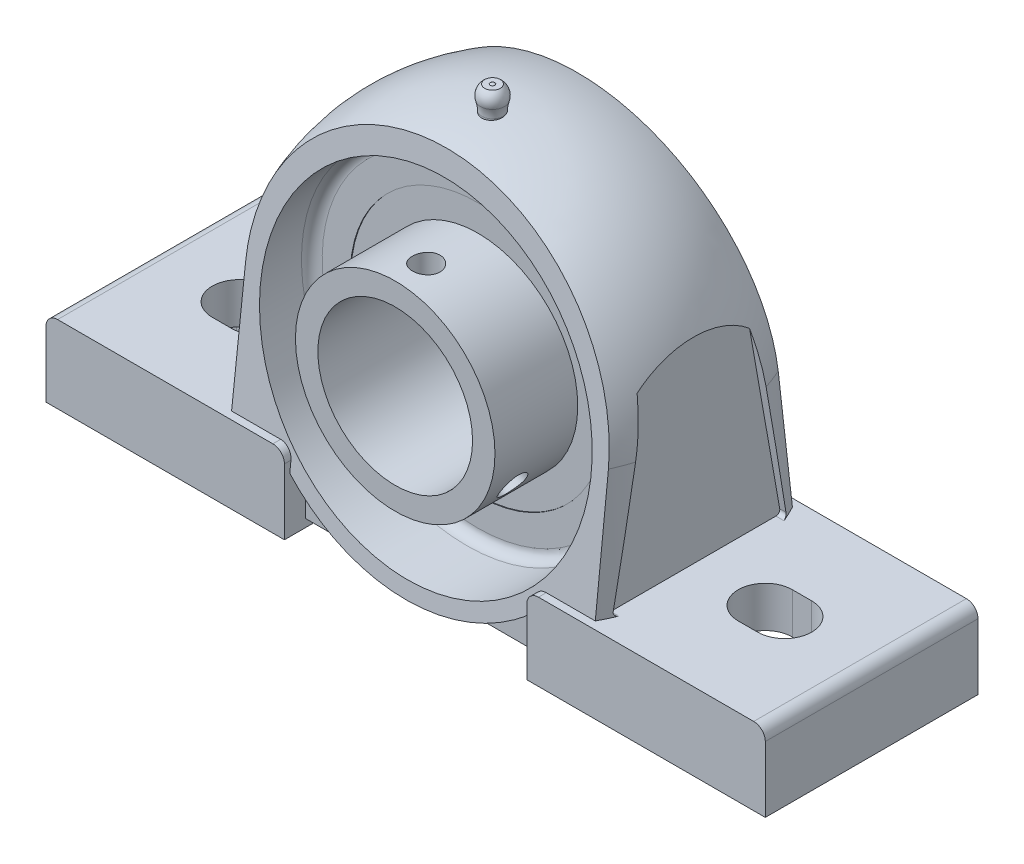
from build123d import *

# Parameters (mm, degrees)
BOSS_EXTRUDE_DEPTH              = 122.2
CUT_EXTRUDE1_DEPTH              = 80.400476324
CUT_EXTRUDE1_DEPTH_BACK         = 80.400476324
SKETCH5_OUTSIDE_W               = 85.446
SKETCH5_OUTSIDE_H               = 131.996
BOSS_EXTRUDE4_REACH             = 85.424
BOSS_EXTRUDE4_DIRECTION_2_REACH = 85.424
BOSS_EXTRUDE1_DEPTH             = 27.5
BOSS_EXTRUDE1_DEPTH_BACK        = 27.5
CUT_EXTRUDE3_DEPTH              = 145.261879946
CUT_EXTRUDE4_DEPTH              = 9.4
CUT_EXTRUDE4_DRAFT              = -1
CUT_EXTRUDE4_PROFILE_2_DEPTH    = 9.4
CUT_EXTRUDE4_PROFILE_2_DRAFT    = -1
CIRPATTERN1_COUNT               = 15
SKETCH14_W                      = 49.2
SKETCH14_H                      = 5.8
SKETCH16_W                      = 3.567
SKETCH16_H                      = 8
SKETCH15_W                      = 0.1
SKETCH15_H                      = 7.42
CIRPATTERN2_COUNT               = 2
CIRPATTERN2_ANGLE               = 120
CUT_EXTRUDE5_START              = 46.88824
CUT_EXTRUDE5_DEPTH              = 7.51176
CUT_EXTRUDE6_START              = -54.4
CUT_EXTRUDE6_DEPTH              = 7.50698


with BuildPart() as part:
    # Sketch1 → Boss-Extrude (new body)
    with BuildSketch(Plane(origin=(0, -47.2, 0), x_dir=(-1, 0, 0), z_dir=(0, 1, 0))):
        with BuildLine():
            Line((-47.716290457, 26.125), (47.716290457, 26.125))
            ThreePointArc((47.716290457, 26.125), (54.4, 0), (47.716290457, -26.125))
            Line((47.716290457, -26.125), (-47.716290457, -26.125))
            ThreePointArc((-47.716290457, -26.125), (-54.4, 0), (-47.716290457, 26.125))
        make_face()
    extrude(amount=BOSS_EXTRUDE_DEPTH)

    # Cut-Sweep1: sweep along a path in Sketch3
    with BuildLine(Plane.XY) as cut_sweep1_path:
        Line((-54.4, -47.2), (-51.514864415, 2.96289458))
        ThreePointArc((-51.514864415, 2.96289458), (0, 51.6), (51.514864415, 2.96289458))
        Line((51.514864415, 2.96289458), (54.4, -47.2))
    # Sketch2 → Cut-Sweep1 (sweep, cut)
    with BuildSketch(Plane(origin=(0, -47.2, 0), x_dir=(-1, 0, 0), z_dir=(0, 1, 0))):
        with BuildLine():
            Line((-47.716290457, 26.125), (-176.6, 26.125))
            Line((-176.6, 26.125), (-176.6, -26.125))
            Line((-176.6, -26.125), (-47.716290457, -26.125))
            ThreePointArc((-47.716290457, -26.125), (-54.4, 0), (-47.716290457, 26.125))
        make_face()
    sweep(path=cut_sweep1_path.line, mode=Mode.SUBTRACT)

    # Sketch5 outside → Cut-Extrude1 (cut, two sides: drawn at the far end of the back side and taken through both)
    with BuildSketch(Plane(origin=(0, 0, 0), x_dir=(0, 0, -1), z_dir=(1, 0, 0)).offset(-CUT_EXTRUDE1_DEPTH_BACK)):
        with Locations((0, 2.2)):
            Rectangle(SKETCH5_OUTSIDE_W, SKETCH5_OUTSIDE_H)
        Polygon((16.5, 52.6), (26.125, -35), (22, -35), (22, -50.2), (-22, -50.2), (-22, -35), (-26.125, -35), (-16.5, 52.6), align=None, mode=Mode.SUBTRACT)
    extrude(amount=CUT_EXTRUDE1_DEPTH + CUT_EXTRUDE1_DEPTH_BACK, mode=Mode.SUBTRACT)

    # Sketch6 → Cut-Revolve2 (revolve, cut)
    with BuildSketch(Plane(origin=(0, 0, 0), x_dir=(0, 0, -1), z_dir=(1, 0, 0)), mode=Mode.PRIVATE) as cut_revolve2_sk:
        with BuildLine():
            Line((-31.413703787, 42.761904762), (-11.679047619, 42.761904762))
            ThreePointArc((-11.679047619, 42.761904762), (-9.78467488, 41.977229881), (-9, 40.082857143))
            Line((-9, 40.082857143), (-9, 38.97435054))
            ThreePointArc((-9, 38.97435054), (-7.684345691, 39.254946584), (-6.36, 39.491143311))
            Line((-6.36, 39.491143311), (-6.36, 42.761904762))
            Line((-6.36, 42.761904762), (-3.72, 42.761904762))
            Line((-3.72, 42.761904762), (-3.72, 39.826644348))
            ThreePointArc((-3.72, 39.826644348), (2.674172991, 39.910509879), (9, 38.97435054))
            Line((9, 38.97435054), (9, 40.082857143))
            ThreePointArc((9, 40.082857143), (9.78467488, 41.977229881), (11.679047619, 42.761904762))
            Line((11.679047619, 42.761904762), (31.413703787, 42.761904762))
            Line((31.413703787, 42.761904762), (36.112143665, 0))
            Line((36.112143665, 0), (-36.112143665, 0))
            Line((-36.112143665, 0), (-31.413703787, 42.761904762))
        make_face()
    revolve(cut_revolve2_sk.sketch.rotate(Axis((0, 0, 0), (0, 0, -1)), 180), axis=Axis((0, 0, 0), (0, 0, -1)), mode=Mode.SUBTRACT)

    # Sketch11 → Boss-Revolve1 (revolve)
    with BuildSketch(Plane.XY.offset(5.04)):
        with BuildLine():
            Line((0, 48.911279127), (0, 57.6))
            ThreePointArc((0, 57.6), (-0.328456711, 57.530107141), (-0.6, 57.332539267))
            Line((-0.6, 57.332539267), (-2, 57.332539267))
            ThreePointArc((-2, 57.332539267), (-3.100653507, 55.744684437), (-3.105555556, 53.812665525))
            ThreePointArc((-3.105555556, 53.812665525), (-2.83938828, 52.646746373), (-2.75, 51.454176785))
            Line((-2.75, 51.454176785), (-2.75, 48.911279127))
            Line((-2.75, 48.911279127), (0, 48.911279127))
        make_face()
    revolve(axis=Axis((0, 0, 5.04), (0, 1, 0)))

    # Boss-Extrude4: up to this plane
    boss_extrude4_end = Plane(origin=(-54.4, 52.6, -16.5), z_dir=(0, 0.10921715097101498, -0.9940179142921794))
    # Sketch9 → Boss-Extrude4 (add, up to the surface)
    with BuildSketch(Plane.XY, mode=Mode.PRIVATE) as boss_extrude4_sk1:
        with BuildLine():
            Line((24.567875343, -35), (31.341433126, -35))
            ThreePointArc((31.341433126, -35), (0, -46.981756357), (-31.341433126, -35))
            Line((-31.341433126, -35), (-24.567875343, -35))
            ThreePointArc((-24.567875343, -35), (0, -42.761904762), (24.567875343, -35))
        make_face()
    boss_extrude4_tool1 = split(extrude(boss_extrude4_sk1.sketch, amount=-BOSS_EXTRUDE4_REACH, mode=Mode.PRIVATE), bisect_by=boss_extrude4_end, keep=Keep.BOTH, mode=Mode.PRIVATE)
    add(boss_extrude4_tool1.solids().sort_by_distance((27.954654, -35.638177, 0))[0])

    # Boss-Extrude4 direction 2: up to this plane
    boss_extrude4_direction_2_end = Plane(origin=(-54.4, 52.6, 16.5), z_dir=(0, 0.10921715097101498, 0.9940179142921794))
    # Sketch9 → Boss-Extrude4 direction 2 (add, up to the surface)
    with BuildSketch(Plane.XY, mode=Mode.PRIVATE) as boss_extrude4_direction_2_sk1:
        with BuildLine():
            Line((24.567875343, -35), (31.341433126, -35))
            ThreePointArc((31.341433126, -35), (0, -46.981756357), (-31.341433126, -35))
            Line((-31.341433126, -35), (-24.567875343, -35))
            ThreePointArc((-24.567875343, -35), (0, -42.761904762), (24.567875343, -35))
        make_face()
    boss_extrude4_direction_2_tool1 = split(extrude(boss_extrude4_direction_2_sk1.sketch, amount=BOSS_EXTRUDE4_DIRECTION_2_REACH, mode=Mode.PRIVATE), bisect_by=boss_extrude4_direction_2_end, keep=Keep.BOTH, mode=Mode.PRIVATE)
    add(boss_extrude4_direction_2_tool1.solids().sort_by_distance((27.954654, -35.638177, 0))[0])

    # Sketch4 → Boss-Extrude1 (add, two sides: drawn at the far end of the back side and taken through both)
    with BuildSketch(Plane.XY.offset(-BOSS_EXTRUDE1_DEPTH_BACK)):
        with BuildLine():
            Line((34.341433126, -29.2), (90, -29.2))
            ThreePointArc((90, -29.2), (92.121320344, -30.078679656), (93, -32.2))
            Line((93, -32.2), (93, -49.2))
            Line((93, -49.2), (31.341433126, -49.2))
            Line((31.341433126, -49.2), (31.341433126, -32.2))
            ThreePointArc((31.341433126, -32.2), (32.220112782, -30.078679656), (34.341433126, -29.2))
        make_face()
        with BuildLine():
            Line((-90, -29.2), (-34.341433126, -29.2))
            ThreePointArc((-34.341433126, -29.2), (-32.220112782, -30.078679656), (-31.341433126, -32.2))
            Line((-31.341433126, -32.2), (-31.341433126, -49.2))
            Line((-31.341433126, -49.2), (-93, -49.2))
            Line((-93, -49.2), (-93, -32.2))
            ThreePointArc((-93, -32.2), (-92.121320344, -30.078679656), (-90, -29.2))
        make_face()
    extrude(amount=BOSS_EXTRUDE1_DEPTH + BOSS_EXTRUDE1_DEPTH_BACK)

    # Sketch7 → Cut-Extrude3 (cut, through all)
    with BuildSketch(Plane.XZ.offset(49.2)):
        with BuildLine():
            Line((-65.5, 7), (-70.5, 7))
            ThreePointArc((-70.5, 7), (-77.5, 0), (-70.5, -7))
            Line((-70.5, -7), (-65.5, -7))
            ThreePointArc((-65.5, -7), (-58.5, 0), (-65.5, 7))
        make_face()
        with BuildLine():
            Line((65.5, -7), (70.5, -7))
            ThreePointArc((70.5, -7), (77.5, 0), (70.5, 7))
            Line((70.5, 7), (65.5, 7))
            ThreePointArc((65.5, 7), (58.5, 0), (65.5, -7))
        make_face()
    extrude(amount=-CUT_EXTRUDE3_DEPTH, mode=Mode.SUBTRACT)


with BuildPart() as cut_extrude4_tool:
    # Sketch10 → Cut-Extrude4 (with draft: the straight prism first)
    with BuildSketch(Plane.XZ.offset(49.2)):
        with BuildLine():
            ThreePointArc((70.5, -14.41), (71.015492065, -13.165492065), (72.26, -12.65))
            Line((72.26, -12.65), (83.815, -12.65))
            ThreePointArc((83.815, -12.65), (85.059507935, -12.134507935), (85.575, -10.89))
            Line((85.575, -10.89), (85.575, 10.89))
            ThreePointArc((85.575, 10.89), (85.059507935, 12.134507935), (83.815, 12.65))
            Line((83.815, 12.65), (72.26, 12.65))
            ThreePointArc((72.26, 12.65), (71.015492065, 13.165492065), (70.5, 14.41))
            Line((70.5, 14.41), (70.5, 18.315))
            ThreePointArc((70.5, 18.315), (69.984507935, 19.559507935), (68.74, 20.075))
            Line((68.74, 20.075), (40.526433126, 20.075))
            ThreePointArc((40.526433126, 20.075), (39.281925191, 19.559507935), (38.766433126, 18.315))
            Line((38.766433126, 18.315), (38.766433126, -18.315))
            ThreePointArc((38.766433126, -18.315), (39.281925191, -19.559507935), (40.526433126, -20.075))
            Line((40.526433126, -20.075), (68.74, -20.075))
            ThreePointArc((68.74, -20.075), (69.984507935, -19.559507935), (70.5, -18.315))
            Line((70.5, -18.315), (70.5, -14.41))
        make_face()
    extrude(amount=-CUT_EXTRUDE4_DEPTH)
    # Cut-Extrude4: the draft: its side faces are tilted about the plane it starts from
    cut_extrude4_sides = [cut_extrude4_tool.faces().sort_by_distance(p)[0] for p in [
        (71.015492065, -44.5, -13.165492065),
        (78.0375, -44.5, -12.65),
        (85.059507935, -44.5, -12.134507935),
        (85.575, -44.5, 0),
        (85.059507935, -44.5, 12.134507935),
        (78.0375, -44.5, 12.65),
        (71.015492065, -44.5, 13.165492065),
        (70.5, -44.5, 16.3625),
        (69.984507935, -44.5, 19.559507935),
        (54.633216563, -44.5, 20.075),
        (39.281925191, -44.5, 19.559507935),
        (38.766433126, -44.5, 0),
        (39.281925191, -44.5, -19.559507935),
        (54.633216563, -44.5, -20.075),
        (69.984507935, -44.5, -19.559507935),
        (70.5, -44.5, -16.3625),
    ]]
    draft(cut_extrude4_sides, Plane.XZ.offset(49.2), CUT_EXTRUDE4_DRAFT)


with BuildPart() as part_1:
    add(part.part)

    # Cut-Extrude4: cut by cut_extrude4_tool
    add(cut_extrude4_tool.part, mode=Mode.SUBTRACT)


with BuildPart() as cut_extrude4_profile_2_tool:
    # Sketch10 → Cut-Extrude4 profile 2 (with draft: the straight prism first)
    with BuildSketch(Plane.XZ.offset(49.2)):
        with BuildLine():
            Line((-83.815, -12.65), (-72.26, -12.65))
            ThreePointArc((-72.26, -12.65), (-71.015492065, -13.165492065), (-70.5, -14.41))
            Line((-70.5, -14.41), (-70.5, -18.315))
            ThreePointArc((-70.5, -18.315), (-69.984507935, -19.559507935), (-68.74, -20.075))
            Line((-68.74, -20.075), (-40.526433126, -20.075))
            ThreePointArc((-40.526433126, -20.075), (-39.281925191, -19.559507935), (-38.766433126, -18.315))
            Line((-38.766433126, -18.315), (-38.766433126, 18.315))
            ThreePointArc((-38.766433126, 18.315), (-39.281925191, 19.559507935), (-40.526433126, 20.075))
            Line((-40.526433126, 20.075), (-68.74, 20.075))
            ThreePointArc((-68.74, 20.075), (-69.984507935, 19.559507935), (-70.5, 18.315))
            Line((-70.5, 18.315), (-70.5, 14.41))
            ThreePointArc((-70.5, 14.41), (-71.015492065, 13.165492065), (-72.26, 12.65))
            Line((-72.26, 12.65), (-83.815, 12.65))
            ThreePointArc((-83.815, 12.65), (-85.059507935, 12.134507935), (-85.575, 10.89))
            Line((-85.575, 10.89), (-85.575, -10.89))
            ThreePointArc((-85.575, -10.89), (-85.059507935, -12.134507935), (-83.815, -12.65))
        make_face()
    extrude(amount=-CUT_EXTRUDE4_PROFILE_2_DEPTH)
    # Cut-Extrude4 profile 2: the draft: its side faces are tilted about the plane it starts from
    cut_extrude4_profile_2_sides = [cut_extrude4_profile_2_tool.faces().sort_by_distance(p)[0] for p in [
        (-78.0375, -44.5, 12.65),
        (-85.059507935, -44.5, 12.134507935),
        (-85.575, -44.5, 0),
        (-85.059507935, -44.5, -12.134507935),
        (-78.0375, -44.5, -12.65),
        (-71.015492065, -44.5, -13.165492065),
        (-70.5, -44.5, -16.3625),
        (-69.984507935, -44.5, -19.559507935),
        (-54.633216563, -44.5, -20.075),
        (-39.281925191, -44.5, -19.559507935),
        (-38.766433126, -44.5, 0),
        (-39.281925191, -44.5, 19.559507935),
        (-54.633216563, -44.5, 20.075),
        (-69.984507935, -44.5, 19.559507935),
        (-70.5, -44.5, 16.3625),
        (-71.015492065, -44.5, 13.165492065),
    ]]
    draft(cut_extrude4_profile_2_sides, Plane.XZ.offset(49.2), CUT_EXTRUDE4_PROFILE_2_DRAFT)


with BuildPart() as part_2:
    add(part_1.part)

    # Cut-Extrude4 profile 2: cut by cut_extrude4_profile_2_tool
    add(cut_extrude4_profile_2_tool.part, mode=Mode.SUBTRACT)

    # Sketch12 → Boss-Revolve3 (revolve)
    with BuildSketch(Plane(origin=(0, 0, 0), x_dir=(0, 0, -1), z_dir=(1, 0, 0)), mode=Mode.PRIVATE) as boss_revolve3_sk:
        with BuildLine():
            Line((9, 38.99435054), (9, 32.82))
            Line((9, 32.82), (-9, 32.82))
            Line((-9, 32.82), (-9, 38.99435054))
            ThreePointArc((-9, 38.99435054), (0, 40.02), (9, 38.99435054))
        make_face()
    revolve(boss_revolve3_sk.sketch.rotate(Axis((0, 0, 0), (0, 0, -1)), 180), axis=Axis((0, 0, 0), (0, 0, -1)))

    # Sketch13 → Boss-Revolve4 (revolve)
    with BuildSketch(Plane(origin=(0, 0, 0), x_dir=(0, 0, -1), z_dir=(1, 0, 0))):
        with BuildLine():
            Line((0, 35.72), (0, 24.32))
            ThreePointArc((0, 24.32), (5.7, 30.02), (0, 35.72))
        make_face()
    boss_revolve4 = revolve(axis=Axis((0, 0, 0), (0, 1, 0)))

    # CirPattern1: Boss-Revolve4 ×15 about axis
    cirpattern1_axis = Axis((0, 0, 0), (0, 0, 1))
    for i in range(1, CIRPATTERN1_COUNT):
        add(boss_revolve4.rotate(cirpattern1_axis, i * 360 / CIRPATTERN1_COUNT))

    # Sketch14 → Boss-Revolve5 (revolve)
    with BuildSketch(Plane(origin=(0, 0, 0), x_dir=(0, 0, -1), z_dir=(1, 0, 0)), mode=Mode.PRIVATE) as boss_revolve5_sk:
        with Locations((-5.6, 22.9)):
            Rectangle(SKETCH14_W, SKETCH14_H)
    revolve(boss_revolve5_sk.sketch.rotate(Axis((0, 0, 0), (0, 0, -1)), 90), axis=Axis((0, 0, 0), (0, 0, -1)))

    # Sketch16 → Cut-Revolve3 (revolve, cut)
    with BuildSketch(Plane(origin=(0, 0, 0), x_dir=(0, 0, -1), z_dir=(1, 0, 0))):
        with Locations((-23.9835, 22)):
            Rectangle(SKETCH16_W, SKETCH16_H)
    cut_revolve3 = revolve(axis=Axis((0, 26, 22.2), (0, -1, 0)), mode=Mode.SUBTRACT)

    # Sketch15 → Boss-Revolve6 (revolve)
    with BuildSketch(Plane(origin=(0, 0, 0), x_dir=(0, 0, -1), z_dir=(1, 0, 0)), mode=Mode.PRIVATE) as boss_revolve6_sk:
        with Locations((-8.75, 29.31)):
            Rectangle(SKETCH15_W, SKETCH15_H)
        with Locations((8.75, 29.31)):
            Rectangle(SKETCH15_W, SKETCH15_H)
    revolve(boss_revolve6_sk.sketch.rotate(Axis((0, 0, 0), (0, 0, -1)), 90), axis=Axis((0, 0, 0), (0, 0, -1)))

    # CirPattern2: Cut-Revolve3 ×2 about axis
    cirpattern2_axis = Axis((0, 0, -21.702927371), (0, 0, -1))
    for i in range(1, CIRPATTERN2_COUNT):
        add(cut_revolve3.rotate(cirpattern2_axis, i * CIRPATTERN2_ANGLE / (CIRPATTERN2_COUNT - 1)), mode=Mode.SUBTRACT)

    # Sketch 17_2 → Cut-Extrude5 (cut)
    with BuildSketch(Plane(origin=(0, 0, 0), x_dir=(0, 0, -1), z_dir=(1, 0, 0)).offset(CUT_EXTRUDE5_START)):
        with BuildLine():
            Line((8.772409121, 48.911279127), (-8.772409121, 48.911279127))
            Line((-8.772409121, 48.911279127), (-22.338589289, -28.026351822))
            ThreePointArc((-22.338589289, -28.026351822), (-22.119825979, -28.84278761), (-21.353781536, -29.2))
            Line((-21.353781536, -29.2), (21.353781536, -29.2))
            ThreePointArc((21.353781536, -29.2), (22.119825979, -28.84278761), (22.338589289, -28.026351822))
            Line((22.338589289, -28.026351822), (8.772409121, 48.911279127))
        make_face()
    extrude(amount=CUT_EXTRUDE5_DEPTH, mode=Mode.SUBTRACT)

    # Sketch 17_2 2 → Cut-Extrude6 (cut)
    with BuildSketch(Plane(origin=(0, 0, 0), x_dir=(0, 0, -1), z_dir=(1, 0, 0)).offset(CUT_EXTRUDE6_START)):
        with BuildLine():
            Line((8.772409121, 48.911279127), (-8.772409121, 48.911279127))
            Line((-8.772409121, 48.911279127), (-22.338589289, -28.026351822))
            ThreePointArc((-22.338589289, -28.026351822), (-22.119825979, -28.84278761), (-21.353781536, -29.2))
            Line((-21.353781536, -29.2), (21.353781536, -29.2))
            ThreePointArc((21.353781536, -29.2), (22.119825979, -28.84278761), (22.338589289, -28.026351822))
            Line((22.338589289, -28.026351822), (8.772409121, 48.911279127))
        make_face()
    extrude(amount=CUT_EXTRUDE6_DEPTH, mode=Mode.SUBTRACT)


solid = part_2.part
